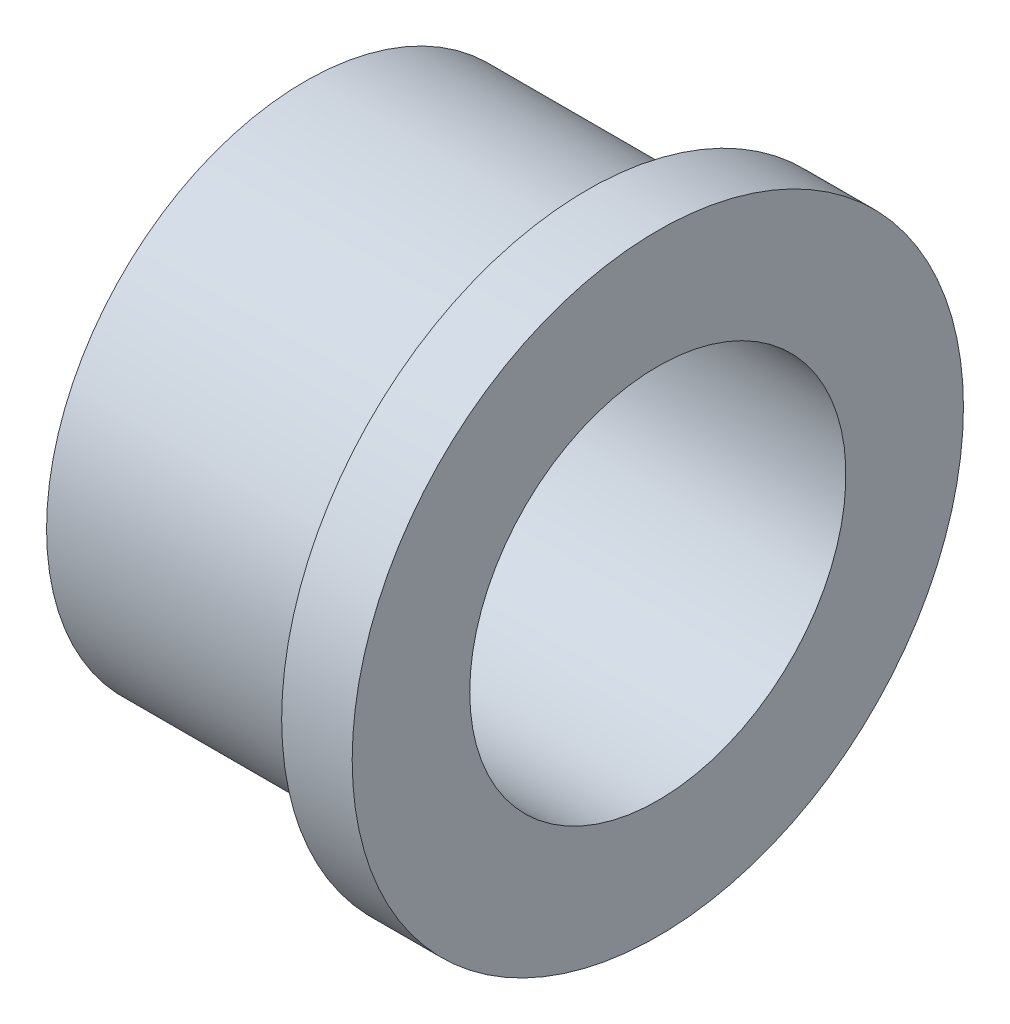
SolidWorks part; units mm, degrees
ref_plane "Front Plane" through (0, 0, 0) normal (0, 0, 1) x (1, 0, 0)
ref_plane "Top Plane" through (0, 0, 0) normal (0, 1, 0) x (1, 0, 0)
ref_plane "Right Plane" through (0, 0, 0) normal (1, 0, 0) x (0, 0, -1)
sketch "Sketch 1" plane through (0, 0, 0) normal (0, 0, 1) x (1, 0, 0)
  line L0 (-54.7855, 0) -> (18.7625, 0) construction
  line L1 (0, 40.2843) -> (0, -50.7692) construction
  line L2 (0, 32.5) -> (0, 20)
  line L3 (0, 20) -> (-37.5, 20)
  line L4 (-37.5, 20) -> (-37.5, 27.5)
  line L5 (-37.5, 27.5) -> (-7.5, 27.5)
  line L6 (-7.5, 27.5) -> (-7.5, 32.5)
  line L7 (-7.5, 32.5) -> (0, 32.5)
  dimension "D1" = 55
  dimension "D2" = 40
  dimension "D3" = 30
  dimension "D4" = 7.5
  dimension "D5" = 5
revolve "Revolve 1" add sketch "Sketch 1" angle 360 about L0
